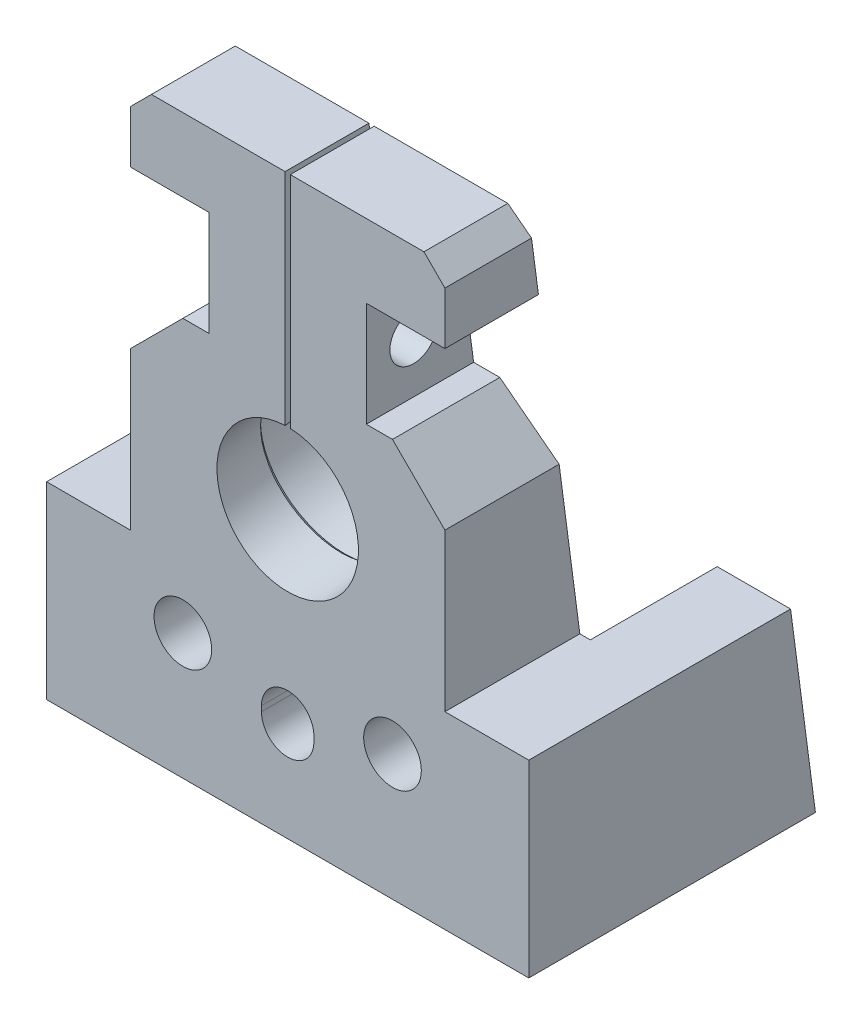
from build123d import *

# Parameters (mm, degrees)
SKETCH1_W                      = 46
SKETCH1_H                      = 55
BOSS_EXTRUDE1_DEPTH            = 20
CUT_EXTRUDE1_DEPTH             = 58.203583804
SKETCH3_R                      = 6.75
CUT_EXTRUDE2_DEPTH             = 47.296696276
SKETCH4_R                      = 2.5
CUT_EXTRUDE3_DEPTH             = 54.714523176
SKETCH6_W                      = 8
SKETCH6_H                      = 37
CUT_EXTRUDE4_DEPTH             = 54.714523176
CUT_EXTRUDE5_DEPTH             = 16
CUT_EXTRUDE6_DEPTH             = 58.203583804
SKETCH9_R                      = 8
CUT_EXTRUDE7_DEPTH             = 7
CHAMFER1_SIZE                  = 2
F_5_5_5_5_DIAMETER_HOLE1_D     = 5.5
SKETCH12_R                     = 4.75
CUT_EXTRUDE8_DEPTH             = 42.723313638
M3_TAPPED_HOLE2_D              = 2.5
M3_TAPPED_HOLE2_DEPTH          = 7.5
M3_TAPPED_HOLE2_TIP            = 0.751075774
SKETCH17_W                     = 0.5
SKETCH17_H                     = 27.5
CUT_EXTRUDE9_DEPTH             = 46.088447741
SKETCH18_W                     = 7.5
SKETCH18_H                     = 10
CUT_EXTRUDE10_DEPTH            = 46.088447741
F_4_5_4_5_DIAMETER_HOLE1_D     = 4.5
F_4_5_4_5_DIAMETER_HOLE1_DEPTH = 7.25
M4_TAPPED_HOLE1_D              = 3.3
M4_TAPPED_HOLE2_D              = 3.3
M4_TAPPED_HOLE2_DEPTH          = 10.1
M4_TAPPED_HOLE2_TIP            = 0.991420021
CHAMFER3_SIZE                  = 5
CHAMFER4_SIZE                  = 0.3
CUT_EXTRUDE11_DEPTH            = 46.088447741


with BuildPart() as part:
    # Sketch1 → Boss-Extrude1 (new, symmetric)
    with BuildSketch(Plane.XY):
        Rectangle(SKETCH1_W, SKETCH1_H)
    extrude(amount=BOSS_EXTRUDE1_DEPTH, both=True)

    # Sketch2 → Cut-Extrude1 (cut, through all)
    with BuildSketch(Plane(origin=(23, 0, 0), x_dir=(0, 0, -1), z_dir=(1, 0, 0))):
        Polygon((-12, 27.5), (20, 27.5), (20, -9.5), (-7.128857589, -9.5), align=None)
    extrude(amount=-CUT_EXTRUDE1_DEPTH, mode=Mode.SUBTRACT)

    # Sketch3 → Cut-Extrude2 (cut, through all)
    with BuildSketch(Plane(origin=(0, -1.084394382, 8.236793088), x_dir=(-1, 0, 0), z_dir=(0, 0.13052619222004844, -0.9914448613738109))):
        with Locations(Location((0, 2.331047994, 0), (0, 0, 90))):
            Circle(SKETCH3_R)
    extrude(amount=-CUT_EXTRUDE2_DEPTH, mode=Mode.SUBTRACT)

    # Sketch4 → Cut-Extrude3 (cut, through all)
    with BuildSketch(Plane.XY.offset(20)):
        with Locations((0, -18)):
            Circle(SKETCH4_R)
    extrude(amount=-CUT_EXTRUDE3_DEPTH, mode=Mode.SUBTRACT)

    # Sketch6 → Cut-Extrude4 (cut, through all)
    with BuildSketch(Plane(origin=(0, 0, -20), x_dir=(-1, 0, 0), z_dir=(0, 0, -1))):
        with Locations((-19, 9)):
            Rectangle(SKETCH6_W, SKETCH6_H)
        with Locations((19, 9)):
            Rectangle(SKETCH6_W, SKETCH6_H)
    extrude(amount=-CUT_EXTRUDE4_DEPTH, mode=Mode.SUBTRACT)

    # Sketch7 → Cut-Extrude5 (cut, symmetric)
    with BuildSketch(Plane(origin=(0, 0, 0), x_dir=(0, 0, -1), z_dir=(1, 0, 0))):
        Polygon((-7.128857589, -9.5), (20, -9.5), (20, -27.5), (-4.759112633, -27.5), align=None)
    extrude(amount=CUT_EXTRUDE5_DEPTH, both=True, mode=Mode.SUBTRACT)

    # Sketch8 → Cut-Extrude6 (cut, through all)
    with BuildSketch(Plane(origin=(23, 0, 0), x_dir=(0, 0, -1), z_dir=(1, 0, 0))):
        Polygon((4.974689938, -9.5), (7.344434894, -27.5), (20, -27.5), (20, -9.5), align=None)
    extrude(amount=-CUT_EXTRUDE6_DEPTH, mode=Mode.SUBTRACT)

    # Sketch9 → Cut-Extrude7 (cut)
    with BuildSketch(Plane(origin=(0, -1.084394382, 8.236793088), x_dir=(-1, 0, 0), z_dir=(0, 0.13052619222004838, -0.9914448613738109))):
        with Locations(Location((0, 2.331047994, 0), (0, 0, 90))):
            Circle(SKETCH9_R)
    extrude(amount=-CUT_EXTRUDE7_DEPTH, mode=Mode.SUBTRACT)

    # Chamfer1
    chamfer1_edges = [part.edges().sort_by_distance(p)[0] for p in [
        (15, 27.5, 16),
        (-15, 27.5, 16),
    ]]
    chamfer(chamfer1_edges, length=CHAMFER1_SIZE)

    # Ø5.5 (5.5) Diameter Hole1 (through all)
    with Locations(Plane.XY.offset(20)):
        with Locations((-10, -15.5), (10, -15.5)):
            Hole(F_5_5_5_5_DIAMETER_HOLE1_D / 2)

    # Sketch12 → Cut-Extrude8 (cut, through all)
    with BuildSketch(Plane.XY.offset(14)):
        with Locations((-10, -15.5)):
            Circle(SKETCH12_R)
        with Locations((10, -15.5)):
            Circle(SKETCH12_R)
    extrude(amount=-CUT_EXTRUDE8_DEPTH, mode=Mode.SUBTRACT)

    # M3 Tapped Hole2
    with Locations(Plane(origin=(0, -1.084394382, 8.236793088), x_dir=(-1, 0, 0), z_dir=(0, 0.13052619222004838, -0.9914448613738109))):
        with Locations((12, 25.831047994), (12, -23.168952006), (-12, -23.168952006)):
            Hole(M3_TAPPED_HOLE2_D / 2, depth=M3_TAPPED_HOLE2_DEPTH)
            with Locations((0, 0, -(M3_TAPPED_HOLE2_DEPTH + M3_TAPPED_HOLE2_TIP / 2))):  # 118° drill point
                Cone(0, M3_TAPPED_HOLE2_D / 2, M3_TAPPED_HOLE2_TIP, mode=Mode.SUBTRACT)

    # Sketch17 → Cut-Extrude9 (cut, through all)
    with BuildSketch(Plane.XY.offset(20)):
        with Locations((0, 13.75)):
            Rectangle(SKETCH17_W, SKETCH17_H)
    extrude(amount=-CUT_EXTRUDE9_DEPTH, mode=Mode.SUBTRACT)

    # Sketch18 → Cut-Extrude10 (cut, through all)
    with BuildSketch(Plane.XY.offset(20)):
        with Locations((-11.25, 15.5)):
            Rectangle(SKETCH18_W, SKETCH18_H)
        with Locations((11.25, 15.5)):
            Rectangle(SKETCH18_W, SKETCH18_H)
    extrude(amount=-CUT_EXTRUDE10_DEPTH, mode=Mode.SUBTRACT)

    # Ø4.5 (4.5) Diameter Hole1
    with Locations(Plane(origin=(7.5, 0, 0), x_dir=(0, 0, -1), z_dir=(1, 0, 0))):
        with Locations((-15.5, 15.5)):
            Hole(F_4_5_4_5_DIAMETER_HOLE1_D / 2, depth=F_4_5_4_5_DIAMETER_HOLE1_DEPTH)

    # M4 Tapped Hole1 (through all)
    with Locations(Plane.ZY.offset(7.5)):
        with Locations((15.5, 15.5)):
            Hole(M4_TAPPED_HOLE1_D / 2)

    # M4 Tapped Hole2
    with Locations(Plane(origin=(0, 0.481919925, -3.660545249), x_dir=(-1, 0, 0), z_dir=(0, 0.13052619222004835, -0.9914448613738109))):
        with Locations((-19, -13.723374809), (-19, -23.723374809), (19, -23.723374809), (19, -13.723374809)):
            Hole(M4_TAPPED_HOLE2_D / 2, depth=M4_TAPPED_HOLE2_DEPTH)
            with Locations((0, 0, -(M4_TAPPED_HOLE2_DEPTH + M4_TAPPED_HOLE2_TIP / 2))):  # 118° drill point
                Cone(0, M4_TAPPED_HOLE2_D / 2, M4_TAPPED_HOLE2_TIP, mode=Mode.SUBTRACT)

    # Chamfer3
    chamfer3_edges = [part.edges().sort_by_distance(p)[0] for p in [
        (-15, 10.5, 14.880953771),
        (15, 10.5, 14.880953771),
    ]]
    chamfer(chamfer3_edges, length=CHAMFER3_SIZE)

    # Chamfer4
    chamfer4_edges = [part.edges().sort_by_distance(p)[0] for p in [
        (0, -6.379224986, 14.600118138),
    ]]
    chamfer(chamfer4_edges, length=CHAMFER4_SIZE)

    # Sketch25 → Cut-Extrude11 (cut, through all)
    with BuildSketch(Plane.XY.offset(20)):
        with BuildLine():
            Line((2.5, -17.75), (2.5, -18.25))
            ThreePointArc((2.5, -18.25), (0, -20.75), (-2.5, -18.25))
            Line((-2.5, -18.25), (-2.5, -17.75))
            ThreePointArc((-2.5, -17.75), (0, -15.25), (2.5, -17.75))
        make_face()
    extrude(amount=-CUT_EXTRUDE11_DEPTH, mode=Mode.SUBTRACT)


solid = part.part
